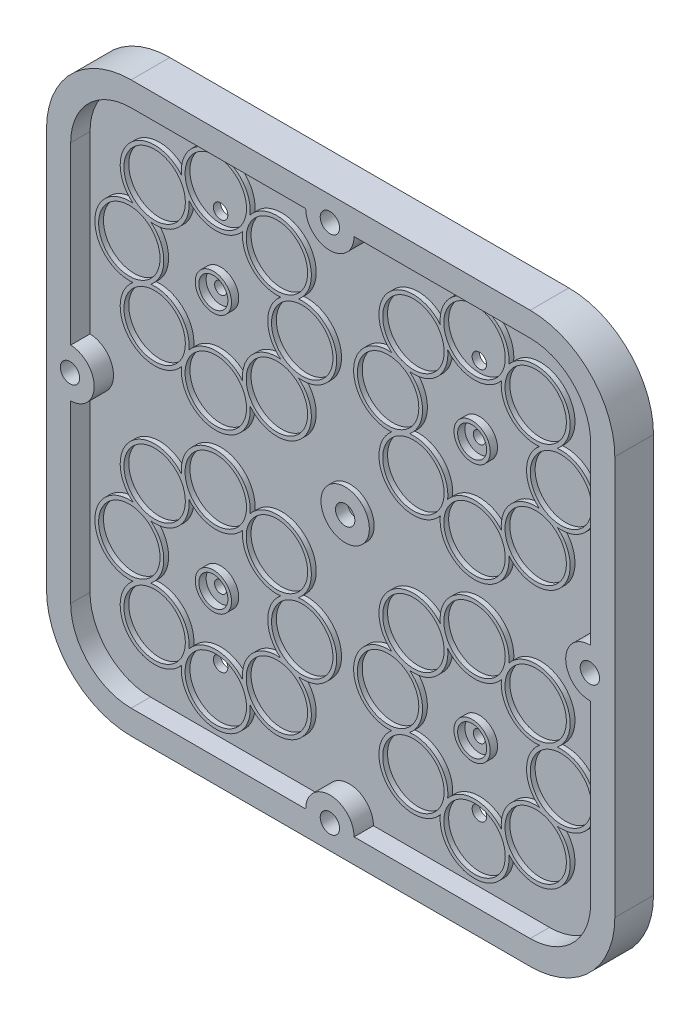
SolidWorks part; units mm, degrees
ref_plane "Front Plane" through (0, 0, 0) normal (0, 0, 1) x (1, 0, 0)
ref_plane "Top Plane" through (0, 0, 0) normal (0, 1, 0) x (1, 0, 0)
ref_plane "Right Plane" through (0, 0, 0) normal (1, 0, 0) x (0, 0, -1)
other "Configuration Table"
sketch "Sketch1" plane through (0, 0, 0) normal (0, 0, 1) x (1, 0, 0)
  line L0 (117.5, 235) -> (117.5, 0) construction
  line L1 (35, 0) -> (200, 0)
  line L2 (0, 35) -> (0, 200)
  line L3 (35, 235) -> (200, 235)
  line L4 (235, 35) -> (235, 200)
  line L5 (0, 117.5) -> (235, 117.5) construction
  line L7 (64, 64) -> (171, 64) construction
  line L8 (64, 64) -> (64, 171) construction
  line L9 (64, 171) -> (171, 171) construction
  line L10 (171, 64) -> (171, 171) construction
  line L11 (64, 64) -> (171, 171) construction
  line L12 (64, 171) -> (171, 64) construction
  arc A0 (200, 0) -> (235, 35) centre (200, 35) ccw
  arc A1 (200, 235) -> (235, 200) centre (200, 200) cw
  arc A2 (35, 0) -> (0, 35) centre (35, 35) cw
  arc A3 (0, 200) -> (35, 235) centre (35, 200) cw
  circle A4 centre (117.5, 225) radius 4
  circle A5 centre (117.5, 10) radius 4
  circle A6 centre (117.5, 117.5) radius 4
  circle A7 centre (225, 117.5) radius 4
  circle A8 centre (10, 117.5) radius 4
  circle A9 centre (64, 171) radius 2.5
  circle A10 centre (171, 171) radius 2.5
  circle A11 centre (171, 64) radius 2.5
  circle A12 centre (64, 64) radius 2.5
  point P7 (235, 0)
  point P12 (0, 0)
  point P15 (0, 235)
  dimension "D3" = 35
  dimension "D4" = 8
  dimension "D5" = 10
  dimension "D6" = 10
  dimension "D7" = 10
  dimension "D8" = 10
  dimension "D11" = 5
  dimension "D1" = 235
  dimension "D2" = 235
  dimension "D9" = 107
  dimension "D10" = 107
extrude "Boss-Extrude1" add sketch "Sketch1" along normal blind 3
sketch "Sketch2" plane through (0, 0, 3) normal (0, 0, 1) x (1, 0, 0)
  line L0 (200, 225) -> (127.186, 225)
  line L1 (10, 200) -> (10, 127.5027)
  line L2 (35, 10) -> (107.186, 10)
  line L3 (225, 35) -> (225, 107.5123)
  line L4 (235, 35) -> (235, 200)
  line L5 (200, 235) -> (35, 235)
  line L6 (0, 200) -> (0, 35)
  line L7 (35, 0) -> (200, 0)
  line L8 (235, 35) -> (235, 200)
  line L9 (200, 235) -> (35, 235)
  line L10 (0, 200) -> (0, 35)
  line L11 (35, 0) -> (200, 0)
  line L12 (10, 107.5104) -> (10, 35)
  line L13 (10, 200) -> (10, 35) construction
  line L14 (107.186, 225) -> (35, 225)
  line L15 (200, 225) -> (35, 225) construction
  line L16 (225, 127.5024) -> (225, 200)
  line L17 (225, 35) -> (225, 200) construction
  line L18 (127.186, 10) -> (200, 10)
  line L19 (35, 10) -> (200, 10) construction
  arc A0 (225, 200) -> (200, 225) centre (200, 200) ccw
  arc A1 (35, 225) -> (10, 200) centre (35, 200) ccw
  arc A2 (10, 35) -> (35, 10) centre (35, 35) ccw
  arc A3 (200, 10) -> (225, 35) centre (200, 35) ccw
  arc A4 (200, 0) -> (235, 35) centre (200, 35) ccw
  arc A5 (235, 200) -> (200, 235) centre (200, 200) ccw
  arc A6 (35, 235) -> (0, 200) centre (35, 200) ccw
  arc A7 (0, 35) -> (35, 0) centre (35, 35) ccw
  arc A8 (200, 0) -> (235, 35) centre (200, 35) ccw
  arc A9 (235, 200) -> (200, 235) centre (200, 200) ccw
  arc A10 (35, 235) -> (0, 200) centre (35, 200) ccw
  arc A11 (0, 35) -> (35, 0) centre (35, 35) ccw
  arc A12 (107.186, 225) -> (127.186, 225) centre (117.186, 225.0074) ccw
  arc A13 (10, 107.5104) -> (10, 127.5027) centre (9.7224, 117.5065) ccw
  arc A15 (225, 127.5024) -> (225, 107.5123) centre (224.686, 117.5074) ccw
  arc A16 (127.186, 10) -> (107.186, 10) centre (117.186, 10.0074) ccw
  circle A17 centre (117.186, 225.0074) radius 4
  circle A18 centre (224.686, 117.5074) radius 4
  circle A19 centre (117.186, 10.0074) radius 4
  circle A20 centre (9.7224, 117.5065) radius 4
  dimension "D1" = 0
  dimension "D2" = 10
extrude "Boss-Extrude2" add sketch "Sketch2" along normal mid plane 16
sketch "Sketch3" plane through (0, 0, 3) normal (0, 0, 1) x (1, 0, 0)
  circle A0 centre (117.5, 117.5) radius 10
  circle A1 centre (117.5, 117.5) radius 4
  dimension "D1" = 20
extrude "Boss-Extrude3" add sketch "Sketch3" along normal blind 2
sketch "Sketch4" plane through (0, 0, 3) normal (0, 0, 1) x (1, 0, 0)
  line L0 (171, 171) -> (171, 221) construction
  circle A2 centre (171, 171) radius 50 construction
  arc A3 (159.8861, 197.8312) -> (182.1139, 197.8312) centre (171, 206.75) ccw
  circle A4 centre (171, 206.75) radius 12.7
  arc A5 (144.1688, 182.1139) -> (159.8861, 197.8312) centre (145.7209, 196.2791) ccw
  circle A6 centre (145.7209, 196.2791) radius 12.7
  arc A7 (136.8021, 185.1652) -> (136.8021, 156.8348) centre (135.25, 171) ccw
  circle A8 centre (135.25, 171) radius 12.7
  arc A9 (159.8861, 144.1688) -> (144.1688, 159.8861) centre (145.7209, 145.7209) ccw
  circle A10 centre (145.7209, 145.7209) radius 12.7
  arc A11 (182.1139, 144.1688) -> (159.8861, 144.1688) centre (171, 135.25) ccw
  circle A12 centre (171, 135.25) radius 12.7
  arc A13 (197.8312, 159.8861) -> (182.1139, 144.1688) centre (196.2791, 145.7209) ccw
  circle A14 centre (196.2791, 145.7209) radius 12.7
  arc A15 (197.8312, 182.1139) -> (197.8312, 159.8861) centre (206.75, 171) ccw
  circle A16 centre (206.75, 171) radius 12.7
  arc A17 (182.1139, 197.8312) -> (197.8312, 182.1139) centre (196.2791, 196.2791) ccw
  circle A18 centre (196.2791, 196.2791) radius 12.7
  arc A19 (156.8348, 205.1979) -> (136.8021, 185.1652) centre (145.7209, 196.2791) ccw
  arc A20 (185.1652, 205.1979) -> (156.8348, 205.1979) centre (171, 206.75) ccw
  arc A21 (205.1979, 185.1652) -> (185.1652, 205.1979) centre (196.2791, 196.2791) ccw
  arc A22 (205.1979, 156.8348) -> (205.1979, 185.1652) centre (206.75, 171) ccw
  arc A23 (185.1652, 136.8021) -> (205.1979, 156.8348) centre (196.2791, 145.7209) ccw
  arc A24 (156.8348, 136.8021) -> (185.1652, 136.8021) centre (171, 135.25) ccw
  arc A25 (144.1688, 159.8861) -> (144.1688, 182.1139) centre (135.25, 171) ccw
  arc A26 (136.8021, 156.8348) -> (156.8348, 136.8021) centre (145.7209, 145.7209) ccw
  circle A27 centre (117.5, 117.5) radius 17.1573 construction
  circle A28 centre (171, 99.75) radius 12.7
  arc A29 (185.1652, 98.1979) -> (156.8348, 98.1979) centre (171, 99.75) ccw
  arc A30 (156.8348, 98.1979) -> (136.8021, 78.1652) centre (145.7209, 89.2791) ccw
  arc A31 (144.1688, 75.1139) -> (159.8861, 90.8312) centre (145.7209, 89.2791) ccw
  arc A32 (159.8861, 90.8312) -> (182.1139, 90.8312) centre (171, 99.75) ccw
  circle A33 centre (145.7209, 89.2791) radius 12.7
  circle A34 centre (135.25, 64) radius 12.7
  arc A35 (144.1688, 52.8861) -> (144.1688, 75.1139) centre (135.25, 64) ccw
  arc A36 (136.8021, 78.1652) -> (136.8021, 49.8348) centre (135.25, 64) ccw
  arc A37 (159.8861, 37.1688) -> (144.1688, 52.8861) centre (145.7209, 38.7209) ccw
  circle A38 centre (145.7209, 38.7209) radius 12.7
  arc A39 (136.8021, 49.8348) -> (156.8348, 29.8021) centre (145.7209, 38.7209) ccw
  arc A40 (156.8348, 29.8021) -> (185.1652, 29.8021) centre (171, 28.25) ccw
  circle A41 centre (171, 28.25) radius 12.7
  arc A42 (182.1139, 37.1688) -> (159.8861, 37.1688) centre (171, 28.25) ccw
  arc A43 (185.1652, 29.8021) -> (205.1979, 49.8348) centre (196.2791, 38.7209) ccw
  circle A44 centre (196.2791, 38.7209) radius 12.7
  arc A45 (197.8312, 52.8861) -> (182.1139, 37.1688) centre (196.2791, 38.7209) ccw
  arc A46 (205.1979, 49.8348) -> (205.1979, 78.1652) centre (206.75, 64) ccw
  circle A47 centre (206.75, 64) radius 12.7
  arc A48 (197.8312, 75.1139) -> (197.8312, 52.8861) centre (206.75, 64) ccw
  arc A49 (182.1139, 90.8312) -> (197.8312, 75.1139) centre (196.2791, 89.2791) ccw
  circle A50 centre (196.2791, 89.2791) radius 12.7
  arc A51 (205.1979, 78.1652) -> (185.1652, 98.1979) centre (196.2791, 89.2791) ccw
  circle A52 centre (99.75, 64) radius 12.7
  arc A53 (98.1979, 49.8348) -> (98.1979, 78.1652) centre (99.75, 64) ccw
  arc A54 (98.1979, 78.1652) -> (78.1652, 98.1979) centre (89.2791, 89.2791) ccw
  arc A55 (75.1139, 90.8312) -> (90.8312, 75.1139) centre (89.2791, 89.2791) ccw
  arc A56 (90.8312, 75.1139) -> (90.8312, 52.8861) centre (99.75, 64) ccw
  circle A57 centre (89.2791, 89.2791) radius 12.7
  circle A58 centre (64, 99.75) radius 12.7
  arc A59 (52.8861, 90.8312) -> (75.1139, 90.8312) centre (64, 99.75) ccw
  arc A60 (78.1652, 98.1979) -> (49.8348, 98.1979) centre (64, 99.75) ccw
  arc A61 (37.1688, 75.1139) -> (52.8861, 90.8312) centre (38.7209, 89.2791) ccw
  circle A62 centre (38.7209, 89.2791) radius 12.7
  arc A63 (49.8348, 98.1979) -> (29.8021, 78.1652) centre (38.7209, 89.2791) ccw
  arc A64 (29.8021, 78.1652) -> (29.8021, 49.8348) centre (28.25, 64) ccw
  circle A65 centre (28.25, 64) radius 12.7
  arc A66 (37.1688, 52.8861) -> (37.1688, 75.1139) centre (28.25, 64) ccw
  arc A67 (29.8021, 49.8348) -> (49.8348, 29.8021) centre (38.7209, 38.7209) ccw
  circle A68 centre (38.7209, 38.7209) radius 12.7
  arc A69 (52.8861, 37.1688) -> (37.1688, 52.8861) centre (38.7209, 38.7209) ccw
  arc A70 (49.8348, 29.8021) -> (78.1652, 29.8021) centre (64, 28.25) ccw
  circle A71 centre (64, 28.25) radius 12.7
  arc A72 (75.1139, 37.1688) -> (52.8861, 37.1688) centre (64, 28.25) ccw
  arc A73 (90.8312, 52.8861) -> (75.1139, 37.1688) centre (89.2791, 38.7209) ccw
  circle A74 centre (89.2791, 38.7209) radius 12.7
  arc A75 (78.1652, 29.8021) -> (98.1979, 49.8348) centre (89.2791, 38.7209) ccw
  circle A76 centre (64, 135.25) radius 12.7
  arc A77 (49.8348, 136.8021) -> (78.1652, 136.8021) centre (64, 135.25) ccw
  arc A78 (78.1652, 136.8021) -> (98.1979, 156.8348) centre (89.2791, 145.7209) ccw
  arc A79 (90.8312, 159.8861) -> (75.1139, 144.1688) centre (89.2791, 145.7209) ccw
  arc A80 (75.1139, 144.1688) -> (52.8861, 144.1688) centre (64, 135.25) ccw
  circle A81 centre (89.2791, 145.7209) radius 12.7
  circle A82 centre (99.75, 171) radius 12.7
  arc A83 (90.8312, 182.1139) -> (90.8312, 159.8861) centre (99.75, 171) ccw
  arc A84 (98.1979, 156.8348) -> (98.1979, 185.1652) centre (99.75, 171) ccw
  arc A85 (75.1139, 197.8312) -> (90.8312, 182.1139) centre (89.2791, 196.2791) ccw
  circle A86 centre (89.2791, 196.2791) radius 12.7
  arc A87 (98.1979, 185.1652) -> (78.1652, 205.1979) centre (89.2791, 196.2791) ccw
  arc A88 (78.1652, 205.1979) -> (49.8348, 205.1979) centre (64, 206.75) ccw
  circle A89 centre (64, 206.75) radius 12.7
  arc A90 (52.8861, 197.8312) -> (75.1139, 197.8312) centre (64, 206.75) ccw
  arc A91 (49.8348, 205.1979) -> (29.8021, 185.1652) centre (38.7209, 196.2791) ccw
  circle A92 centre (38.7209, 196.2791) radius 12.7
  arc A93 (37.1688, 182.1139) -> (52.8861, 197.8312) centre (38.7209, 196.2791) ccw
  arc A94 (29.8021, 185.1652) -> (29.8021, 156.8348) centre (28.25, 171) ccw
  circle A95 centre (28.25, 171) radius 12.7
  arc A96 (37.1688, 159.8861) -> (37.1688, 182.1139) centre (28.25, 171) ccw
  arc A97 (52.8861, 144.1688) -> (37.1688, 159.8861) centre (38.7209, 145.7209) ccw
  circle A98 centre (38.7209, 145.7209) radius 12.7
  arc A99 (29.8021, 156.8348) -> (49.8348, 136.8021) centre (38.7209, 145.7209) ccw
  dimension "D1" = 4
  dimension "D3" = 100
  dimension "D4" = 28.5
  dimension "D5" = 25.4
  dimension "D6" = 8
extrude "Boss-Extrude4" add sketch "Sketch4" along normal blind 2
sketch "Sketch5" plane through (0, 0, 3) normal (0, 0, 1) x (1, 0, 0)
  circle A0 centre (171, 171) radius 6
  circle A1 centre (171, 171) radius 7.5
  circle A2 centre (64, 171) radius 7.5
  circle A3 centre (64, 171) radius 6
  circle A4 centre (64, 64) radius 7.5
  circle A5 centre (64, 64) radius 6
  circle A6 centre (171, 64) radius 7.5
  circle A7 centre (171, 64) radius 6
  dimension "D1" = 12
  dimension "D2" = 15
extrude "Boss-Extrude5" add sketch "Sketch5" along normal blind 3
sketch "Sketch6" plane through (0, 0, 0) normal (0, 0, -1) x (-1, 0, 0)
  line L1 (-64, 36.5) -> (-171, 36.5) construction
  line L2 (-64, 36.5) -> (-64, 198.5) construction
  line L3 (-64, 198.5) -> (-171, 198.5) construction
  line L4 (-171, 36.5) -> (-171, 198.5) construction
  circle A0 centre (-117.5, 117.5) radius 4 construction
  circle A1 centre (-171, 64) radius 2.5 construction
  circle A2 centre (-171, 171) radius 2.5 construction
  circle A3 centre (-64, 36.5) radius 3
  circle A4 centre (-171, 36.5) radius 3
  circle A5 centre (-171, 198.5) radius 3
  circle A6 centre (-64, 198.5) radius 3
  dimension "D3" = 27.5
  dimension "D5" = 6
  dimension "D1" = 107
  dimension "D2" = 53.5
  dimension "D4" = 27.5
extrude "Cut-Extrude1" cut sketch "Sketch6" against normal blind 10
sketch "Sketch7" plane through (0, 0, 0) normal (0, 0, -1) x (-1, 0, 0)
  line L0 (-117.5, 117.5) -> (-117.5, 39.4791) construction
  line L1 (-117.5, 117.5) -> (-187.8752, 117.5) construction
  circle A0 centre (-171, 36.5) radius 19
  arc A1 (-177.9773, 56.8364) -> (-164.0227, 56.8364) centre (-171, 36.5) ccw
  circle A12 centre (-171, 64) radius 7.5
  arc A13 (-164.0227, 56.8364) -> (-177.9773, 56.8364) centre (-171, 64) ccw
  arc A14 (-70.9773, 56.8364) -> (-57.0227, 56.8364) centre (-64, 64) cw
  circle A15 centre (-64, 64) radius 7.5
  arc A16 (-57.0227, 56.8364) -> (-70.9773, 56.8364) centre (-64, 36.5) cw
  circle A17 centre (-64, 36.5) radius 19
  arc A18 (-164.0227, 178.1636) -> (-177.9773, 178.1636) centre (-171, 171) cw
  circle A19 centre (-171, 171) radius 7.5
  arc A20 (-177.9773, 178.1636) -> (-164.0227, 178.1636) centre (-171, 198.5) cw
  circle A21 centre (-171, 198.5) radius 19
  circle A22 centre (-64, 198.5) radius 19
  arc A23 (-57.0227, 178.1636) -> (-70.9773, 178.1636) centre (-64, 198.5) ccw
  circle A24 centre (-64, 171) radius 7.5
  arc A25 (-70.9773, 178.1636) -> (-57.0227, 178.1636) centre (-64, 171) ccw
  dimension "D1" = 38
  dimension "D2" = 43
  dimension "D3" = 15
  dimension "D4" = 20
extrude "Boss-Extrude6" add sketch "Sketch7" along normal blind 4
sketch "Sketch8" plane through (0, 0, 0) normal (0, 0, -1) x (-1, 0, 0)
  circle A0 centre (-117.5, 117.5) radius 9.5
  circle A1 centre (-117.5, 117.5) radius 14.5
  dimension "D1" = 19
  dimension "D2" = 29
extrude "Boss-Extrude7" add sketch "Sketch8" along normal blind 6
